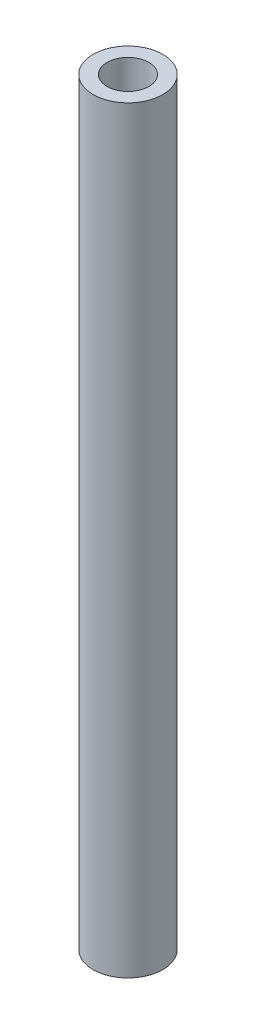
SolidWorks part; units mm, degrees
ref_plane "Front Plane" through (0, 0, 0) normal (0, 0, 1) x (1, 0, 0)
ref_plane "Top Plane" through (0, 0, 0) normal (0, 1, 0) x (1, 0, 0)
ref_plane "Right Plane" through (0, 0, 0) normal (1, 0, 0) x (0, 0, -1)
sketch "Sketch1" plane through (0, 0, 0) normal (0, 1, 0) x (1, 0, 0)
  circle A0 centre (0, 0) radius 2.5
  circle A1 centre (0, 0) radius 1.5
  dimension "D1" = 5
  dimension "D2" = 3
extrude "Boss-Extrude1" add sketch "Sketch1" along normal blind 54.4
cosmetic thread "Cosmetic Thread1" parameters "D1"=5, "D2"=4
sketch "Sketch2" plane through (0, 0, 0) normal (0, -1, 0) x (1, 0, 0)
  circle A0 centre (0, 0) radius 1.5 construction
  circle A1 centre (0, 0) radius 1.5
  circle A2 centre (0, 0) radius 0.5
  dimension "D1" = 1
extrude "Boss-Extrude2" add sketch "Sketch2" against normal blind 2
